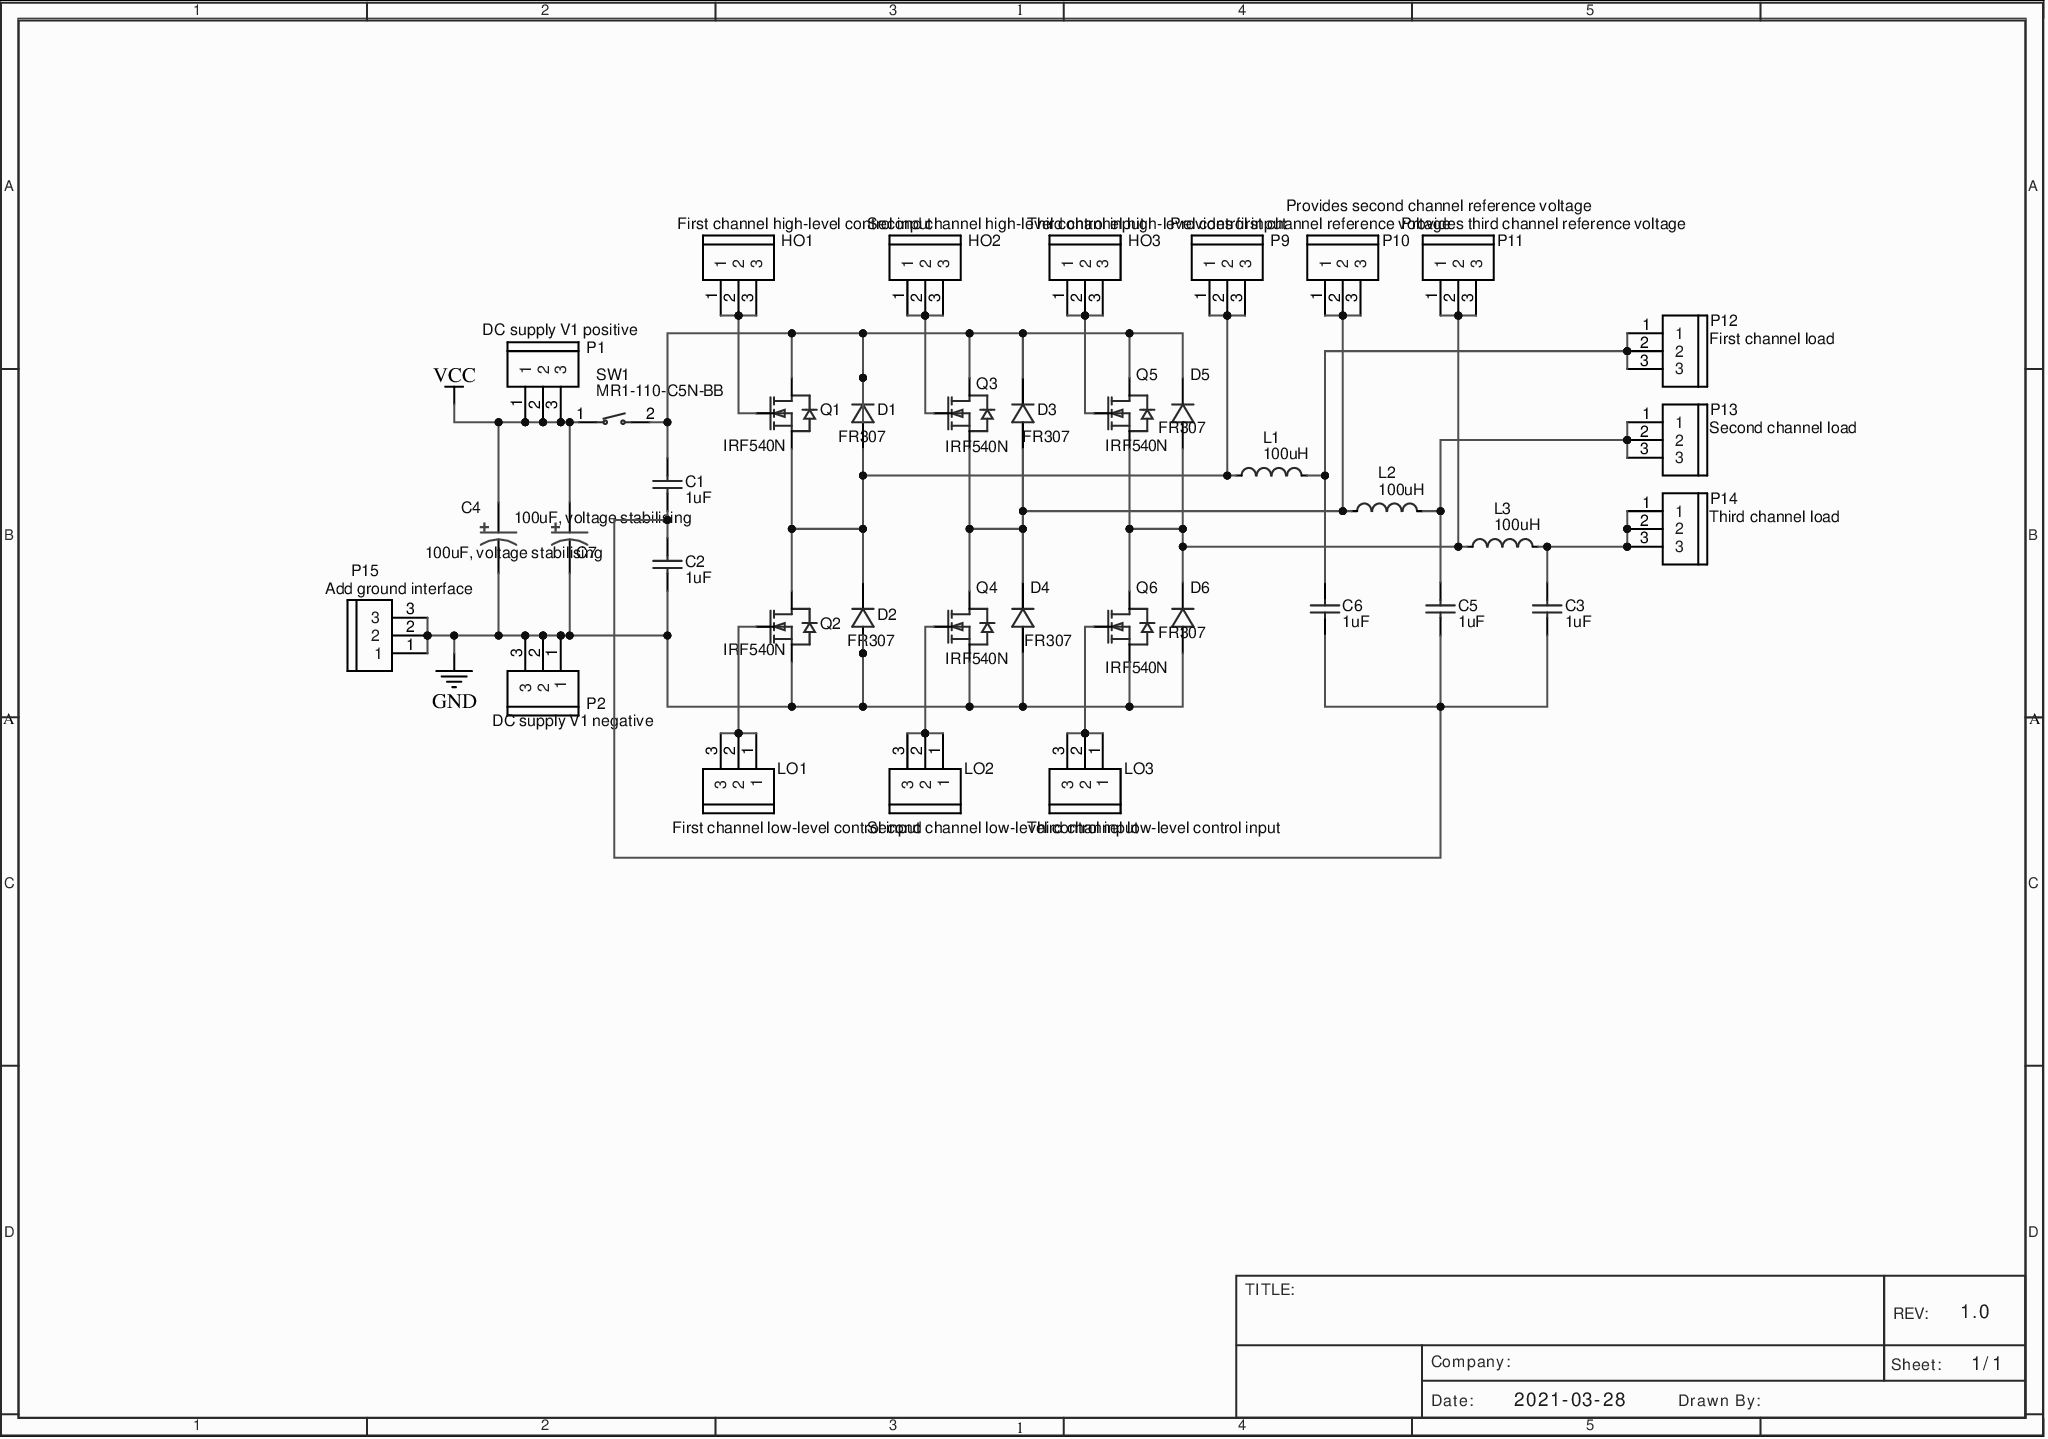
[diagram p0: MISC75150-3.schdoc]
# Altium project MISC75150-2.PrjPcb
1 sheet, 38 parts. Net scope: global (net labels, ports and power ports of the same name join across sheets).
Board file: MISC75150.pcbdoc

## Sheet MISC75150-3.schdoc
size 292 x 205 mm; Name: MISC75150; @Project Name: MISC75150; REV: 1.0; Date: 2021-03-28; Sheet: 1/1; Manufacturer Part: ?

### Parts
C1  1uF  [CAP-TH_L18.0-W9.5-P15.00-D1.2]
C2  1uF  [CAP-TH_L18.0-W9.5-P15.00-D1.2]
C3  1uF  [CAP-TH_L18.0-W9.5-P15.00-D1.2]
C4  100uF, voltage stabilising  [CAP-TH_BD8.0-P3.50-D1.0-FD]
C5  1uF  [CAP-TH_L18.0-W9.5-P15.00-D1.2]
C6  1uF  [CAP-TH_L18.0-W9.5-P15.00-D1.2]
C7  100uF, voltage stabilising  [CAP-TH_BD8.0-P3.50-D1.0-FD]
D1  FR307  [DO-201AD_BD5.3-L8.4-P12.50-D1.4-RD]
D2  FR307  [DO-201AD_BD5.3-L8.4-P12.50-D1.4-RD]
D3  FR307  [DO-201AD_BD5.3-L8.4-P12.50-D1.4-RD]
D4  FR307  [DO-201AD_BD5.3-L8.4-P12.50-D1.4-RD]
D5  FR307  [DO-201AD_BD5.3-L8.4-P12.50-D1.4-RD]
D6  FR307  [DO-201AD_BD5.3-L8.4-P12.50-D1.4-RD]
HO1  First channel high-level control input  [CONN-TH_3P-P5.00_WJ500V-5.08-3P]
HO2  Second channel high-level control input  [CONN-TH_3P-P5.00_WJ500V-5.08-3P]
HO3  Third channel high-level control input  [CONN-TH_3P-P5.00_WJ500V-5.08-3P]
L1  100uH  [IND-SMD_L13.5-W12.6_125CDMCC-DS]
L2  100uH  [IND-SMD_L13.5-W12.6_125CDMCC-DS]
L3  100uH  [IND-SMD_L13.5-W12.6_125CDMCC-DS]
LO1  First channel low-level control input  [CONN-TH_3P-P5.00_WJ500V-5.08-3P]
LO2  Second channel low-level control input  [CONN-TH_3P-P5.00_WJ500V-5.08-3P]
LO3  Third channel low-level control input  [CONN-TH_3P-P5.00_WJ500V-5.08-3P]
P1  DC supply V1 positive  [CONN-TH_3P-P5.00_WJ500V-5.08-3P]
P2  DC supply V1 negative  [CONN-TH_3P-P5.00_WJ500V-5.08-3P]
P9  Provides first channel reference voltage  [CONN-TH_3P-P5.00_WJ500V-5.08-3P]
P10  Provides second channel reference voltage  [CONN-TH_3P-P5.00_WJ500V-5.08-3P]
P11  Provides third channel reference voltage  [CONN-TH_3P-P5.00_WJ500V-5.08-3P]
P12  First channel load  [CONN-TH_3P-P5.00_WJ500V-5.08-3P]
P13  Second channel load  [CONN-TH_3P-P5.00_WJ500V-5.08-3P]
P14  Third channel load  [CONN-TH_3P-P5.00_WJ500V-5.08-3P]
P15  Add ground interface  [CONN-TH_3P-P5.00_WJ500V-5.08-3P]
Q1  IRF540N  [TO-220AB-3_L10.4-W4.6-P2.54-L]
Q2  IRF540N  [TO-220AB-3_L10.4-W4.6-P2.54-L]
Q3  IRF540N  [TO-220AB-3_L10.4-W4.6-P2.54-L]
Q4  IRF540N  [TO-220AB-3_L10.4-W4.6-P2.54-L]
Q5  IRF540N  [TO-220AB-3_L10.4-W4.6-P2.54-L]
Q6  IRF540N  [TO-220AB-3_L10.4-W4.6-P2.54-L]
SW1  MR1-110-C5N-BB  [SW-TH_MR1-110-C5N-BB]

### Nets
GND: C2.1 C4.2 C7.2 D2.2 D4.2 D6.2 P2.1 P2.2 P2.3 P15.1 P15.2 P15.3 Q2.3(S) Q4.3(S) Q6.3(S)
VCC: C4.1 C7.1 P1.1 P1.2 P1.3 SW1.1
NetC1_1: C1.1 C2.2 C3.1 C5.1 C6.1
NetC1_2: C1.2 D1.1 D3.1 D5.1 Q1.2(D) Q3.2(D) Q5.2(D) SW1.2
NetC3_2: C3.2 L3.2 P14.1 P14.2 P14.3
NetC5_2: C5.2 L2.2 P13.1 P13.2 P13.3
NetC6_2: C6.2 L1.2 P12.1 P12.2 P12.3
NetD1_2: D1.2 D2.1 L1.1 P9.1 P9.2 P9.3 Q1.3(S) Q2.2(D)
NetD3_2: D3.2 D4.1 L2.1 P10.1 P10.2 P10.3 Q3.3(S) Q4.2(D)
NetD5_2: D5.2 D6.1 L3.1 P11.1 P11.2 P11.3 Q5.3(S) Q6.2(D)
NetHO1_1: HO1.1 HO1.2 HO1.3 Q1.1(G)
NetHO2_1: HO2.1 HO2.2 HO2.3 Q3.1(G)
NetHO3_1: HO3.1 HO3.2 HO3.3 Q5.1(G)
NetLO1_1: LO1.1 LO1.2 LO1.3 Q2.1(G)
NetLO2_1: LO2.1 LO2.2 LO2.3 Q4.1(G)
NetLO3_1: LO3.1 LO3.2 LO3.3 Q6.1(G)

### Notes on the sheet
- 1
- 2
- 3
- 4
- 5
- A
- B
- C
- D
- TITLE:
- Company:
- Sheet:
- REV:
- 1.0
- 1/1
- Date:
- 2021-03-28
- Drawn By:

### Library data of the parts
C1 = ECWF2W105KA: Manufacturer: PANASONIC; Paste Type: expand; Convert to PCB: yes; UniqueId: ggee4a7045e9711cf46; OriginModelName: CAP-TH_L18.1-W9.3-H12.6-P15.0; ModelTransform: 712.597,366.141,0,0,0,0,0,0,-137.795; Device: ECWF2W105KA; Supplier: LCSC; Manufacturer Part: ECWF2W105KA; Supplier Part: C128505; Add into BOM: yes; SymbolName: 1uF; FootprintName: CAP-TH_L18.0-W9.5-P15.00-D1.2
C2 = ECWF2W105KA: Manufacturer: PANASONIC; Paste Type: expand; Convert to PCB: yes; UniqueId: gge8b30a07ac08630fb; OriginModelName: CAP-TH_L18.1-W9.3-H12.6-P15.0; ModelTransform: 712.597,366.141,0,0,0,0,0,0,-137.795; Device: ECWF2W105KA; Supplier: LCSC; Manufacturer Part: ECWF2W105KA; Supplier Part: C128505; Add into BOM: yes; SymbolName: 1uF; FootprintName: CAP-TH_L18.0-W9.5-P15.00-D1.2
C3 = ECWF2W105KA: Manufacturer: PANASONIC; Paste Type: expand; Convert to PCB: yes; UniqueId: ggeb8cf41ff4f0b6587; OriginModelName: CAP-TH_L18.1-W9.3-H12.6-P15.0; ModelTransform: 712.597,366.141,0,0,0,0,0,0,-137.795; Device: ECWF2W105KA; Supplier: LCSC; Manufacturer Part: ECWF2W105KA; Supplier Part: C128505; Add into BOM: yes; SymbolName: 1uF; FootprintName: CAP-TH_L18.0-W9.5-P15.00-D1.2
C4 = SPV1HM101F11O00RAXXX: Manufacturer: Aihua Group; Convert to PCB: yes; UniqueId: ggee92f5958b3224aee; OriginModelName: CAP-TH_D8.0-H8.0-P3.50; ModelTransform: 314.96,314.862,0,180,0,0,0,0,-118.11; Device: SPV1HM101F11O00RAXXX; Supplier: LCSC; Supplier Part: C167234; Manufacturer Part: SPV1HM101F11O00RAXXX; Add into BOM: yes; SymbolName: 100uF, voltage stabilising; FootprintName: CAP-TH_BD8.0-P3.50-D1.0-FD
C5 = ECWF2W105KA: Manufacturer: PANASONIC; Paste Type: expand; Convert to PCB: yes; UniqueId: gge1386f1878ac6b3a8; OriginModelName: CAP-TH_L18.1-W9.3-H12.6-P15.0; ModelTransform: 712.597,366.141,0,0,0,0,0,0,-137.795; Device: ECWF2W105KA; Supplier: LCSC; Manufacturer Part: ECWF2W105KA; Supplier Part: C128505; Add into BOM: yes; SymbolName: 1uF; FootprintName: CAP-TH_L18.0-W9.5-P15.00-D1.2
C6 = ECWF2W105KA: Manufacturer: PANASONIC; Paste Type: expand; Convert to PCB: yes; UniqueId: gge8976a15bcc07fff3; OriginModelName: CAP-TH_L18.1-W9.3-H12.6-P15.0; ModelTransform: 712.597,366.141,0,0,0,0,0,0,-137.795; Device: ECWF2W105KA; Supplier: LCSC; Manufacturer Part: ECWF2W105KA; Supplier Part: C128505; Add into BOM: yes; SymbolName: 1uF; FootprintName: CAP-TH_L18.0-W9.5-P15.00-D1.2
C7 = SPV1HM101F11O00RAXXX: Manufacturer: Aihua Group; Convert to PCB: yes; UniqueId: ggeb1f74c670b6129be; OriginModelName: CAP-TH_D8.0-H8.0-P3.50; ModelTransform: 314.96,314.862,0,180,0,0,0,0,-118.11; Device: SPV1HM101F11O00RAXXX; Supplier: LCSC; Supplier Part: C167234; Manufacturer Part: SPV1HM101F11O00RAXXX; Add into BOM: yes; SymbolName: 100uF, voltage stabilising; FootprintName: CAP-TH_BD8.0-P3.50-D1.0-FD
D1 = FR307: Manufacturer: Yangzhou Yangjie Elec Tech; Paste Type: expand; Convert to PCB: yes; UniqueId: gge83b63f64a46c2831; OriginModelName: DO-201AD_D5.3-L8.4-P13.6; ModelTransform: 582.676,208.5295,0,0,0,0,0,0,-137.795; Device: FR307; Supplier: LCSC; Supplier Part: C698674; Manufacturer Part: FR307; Add into BOM: yes; SymbolName: FR307; FootprintName: DO-201AD_BD5.3-L8.4-P12.50-D1.4-RD
D2 = FR307: Manufacturer: Yangzhou Yangjie Elec Tech; Paste Type: expand; Convert to PCB: yes; UniqueId: ggea2ef0e735770ea0f; OriginModelName: DO-201AD_D5.3-L8.4-P13.6; ModelTransform: 582.676,208.5295,0,0,0,0,0,0,-137.795; Device: FR307; Supplier: LCSC; Supplier Part: C698674; Manufacturer Part: FR307; Add into BOM: yes; SymbolName: FR307; FootprintName: DO-201AD_BD5.3-L8.4-P12.50-D1.4-RD
D3 = FR307: Manufacturer: Yangzhou Yangjie Elec Tech; Paste Type: expand; Convert to PCB: yes; UniqueId: ggeac6837f34457c33d; OriginModelName: DO-201AD_D5.3-L8.4-P13.6; ModelTransform: 582.676,208.5295,0,0,0,0,0,0,-137.795; Device: FR307; Supplier: LCSC; Supplier Part: C698674; Manufacturer Part: FR307; Add into BOM: yes; SymbolName: FR307; FootprintName: DO-201AD_BD5.3-L8.4-P12.50-D1.4-RD
D4 = FR307: Manufacturer: Yangzhou Yangjie Elec Tech; Paste Type: expand; Convert to PCB: yes; UniqueId: gge96a78163855c4fac; OriginModelName: DO-201AD_D5.3-L8.4-P13.6; ModelTransform: 582.676,208.5295,0,0,0,0,0,0,-137.795; Device: FR307; Supplier: LCSC; Supplier Part: C698674; Manufacturer Part: FR307; Add into BOM: yes; SymbolName: FR307; FootprintName: DO-201AD_BD5.3-L8.4-P12.50-D1.4-RD
D5 = FR307: Manufacturer: Yangzhou Yangjie Elec Tech; Paste Type: expand; Convert to PCB: yes; UniqueId: gge21288790032872b2; OriginModelName: DO-201AD_D5.3-L8.4-P13.6; ModelTransform: 582.676,208.5295,0,0,0,0,0,0,-137.795; Device: FR307; Supplier: LCSC; Supplier Part: C698674; Manufacturer Part: FR307; Add into BOM: yes; SymbolName: FR307; FootprintName: DO-201AD_BD5.3-L8.4-P12.50-D1.4-RD
D6 = FR307: Manufacturer: Yangzhou Yangjie Elec Tech; Paste Type: expand; Convert to PCB: yes; UniqueId: gge82c1ee6ae88ddc6b; OriginModelName: DO-201AD_D5.3-L8.4-P13.6; ModelTransform: 582.676,208.5295,0,0,0,0,0,0,-137.795; Device: FR307; Supplier: LCSC; Supplier Part: C698674; Manufacturer Part: FR307; Add into BOM: yes; SymbolName: FR307; FootprintName: DO-201AD_BD5.3-L8.4-P12.50-D1.4-RD
HO1 = WJ500V-5.08-3P-14-00A: Manufacturer: ReliaPro; Paste Type: expand; Convert to PCB: yes; UniqueId: gge2b5cea29c56c81ac; OriginModelName: CONN-TH_3P_L15.3-W10.2-P5.08; ModelTransform: 619.674,413.385,0,0,0,0,-7.874,0,-157.48; Device: WJ500V-5.08-3P-14-00A; Supplier: LCSC; Manufacturer Part: WJ500V-5.08-3P-14-00A; image: C72334.jpg; Supplier Part: C72334; Add into BOM: yes; SymbolName: First channel high-level control input; FootprintName: CONN-TH_3P-P5.00_WJ500V-5.08-3P
HO2 = WJ500V-5.08-3P-14-00A: Manufacturer: ReliaPro; Paste Type: expand; Convert to PCB: yes; UniqueId: gge3b87de472fa51f12; OriginModelName: CONN-TH_3P_L15.3-W10.2-P5.08; ModelTransform: 619.674,413.385,0,0,0,0,-7.874,0,-157.48; Device: WJ500V-5.08-3P-14-00A; Supplier: LCSC; Manufacturer Part: WJ500V-5.08-3P-14-00A; image: C72334.jpg; Supplier Part: C72334; Add into BOM: yes; SymbolName: Second channel high-level control input; FootprintName: CONN-TH_3P-P5.00_WJ500V-5.08-3P
HO3 = WJ500V-5.08-3P-14-00A: Manufacturer: ReliaPro; Paste Type: expand; Convert to PCB: yes; UniqueId: ggef853e3d0681c0b1a; OriginModelName: CONN-TH_3P_L15.3-W10.2-P5.08; ModelTransform: 619.674,413.385,0,0,0,0,-7.874,0,-157.48; Device: WJ500V-5.08-3P-14-00A; Supplier: LCSC; Manufacturer Part: WJ500V-5.08-3P-14-00A; image: C72334.jpg; Supplier Part: C72334; Add into BOM: yes; SymbolName: Third channel high-level control input; FootprintName: CONN-TH_3P-P5.00_WJ500V-5.08-3P
L1 = TMPC1206HP-101MG-D: Manufacturer: TAITEC; Convert to PCB: yes; UniqueId: gged90d88dc2415983d; OriginModelName: IND-SMD_L13.5-W12.6-H5.7; ModelTransform: 531.495,492.125,0,0,0,0,0,0,0; Device: TMPC1206HP-101MG-D; Supplier: LCSC; Supplier Part: C357256; Manufacturer Part: TMPC1206HP-101MG-D; Add into BOM: yes; SymbolName: 100uH; FootprintName: IND-SMD_L13.5-W12.6_125CDMCC-DS
L2 = TMPC1206HP-101MG-D: Manufacturer: TAITEC; Convert to PCB: yes; UniqueId: ggeadd428e7fae9a274; OriginModelName: IND-SMD_L13.5-W12.6-H5.7; ModelTransform: 531.495,492.125,0,0,0,0,0,0,0; Device: TMPC1206HP-101MG-D; Supplier: LCSC; Supplier Part: C357256; Manufacturer Part: TMPC1206HP-101MG-D; Add into BOM: yes; SymbolName: 100uH; FootprintName: IND-SMD_L13.5-W12.6_125CDMCC-DS
L3 = TMPC1206HP-101MG-D: Manufacturer: TAITEC; Convert to PCB: yes; UniqueId: ggeea68f54d1f5691be; OriginModelName: IND-SMD_L13.5-W12.6-H5.7; ModelTransform: 531.495,492.125,0,0,0,0,0,0,0; Device: TMPC1206HP-101MG-D; Supplier: LCSC; Supplier Part: C357256; Manufacturer Part: TMPC1206HP-101MG-D; Add into BOM: yes; SymbolName: 100uH; FootprintName: IND-SMD_L13.5-W12.6_125CDMCC-DS
LO1 = WJ500V-5.08-3P-14-00A: Manufacturer: ReliaPro; Paste Type: expand; Convert to PCB: yes; UniqueId: gge8d9840f4034438ff; OriginModelName: CONN-TH_3P_L15.3-W10.2-P5.08; ModelTransform: 619.674,413.385,0,0,0,0,-7.874,0,-157.48; Device: WJ500V-5.08-3P-14-00A; Supplier: LCSC; Manufacturer Part: WJ500V-5.08-3P-14-00A; image: C72334.jpg; Supplier Part: C72334; Add into BOM: yes; SymbolName: First channel low-level control input; FootprintName: CONN-TH_3P-P5.00_WJ500V-5.08-3P
LO2 = WJ500V-5.08-3P-14-00A: Manufacturer: ReliaPro; Paste Type: expand; Convert to PCB: yes; UniqueId: gge5f0c870194b11f33; OriginModelName: CONN-TH_3P_L15.3-W10.2-P5.08; ModelTransform: 619.674,413.385,0,0,0,0,-7.874,0,-157.48; Device: WJ500V-5.08-3P-14-00A; Supplier: LCSC; Manufacturer Part: WJ500V-5.08-3P-14-00A; image: C72334.jpg; Supplier Part: C72334; Add into BOM: yes; SymbolName: Second channel low-level control input; FootprintName: CONN-TH_3P-P5.00_WJ500V-5.08-3P
LO3 = WJ500V-5.08-3P-14-00A: Manufacturer: ReliaPro; Paste Type: expand; Convert to PCB: yes; UniqueId: gge96ab42e47ac765f7; OriginModelName: CONN-TH_3P_L15.3-W10.2-P5.08; ModelTransform: 619.674,413.385,0,0,0,0,-7.874,0,-157.48; Device: WJ500V-5.08-3P-14-00A; Supplier: LCSC; Manufacturer Part: WJ500V-5.08-3P-14-00A; image: C72334.jpg; Supplier Part: C72334; Add into BOM: yes; SymbolName: Third channel low-level control input; FootprintName: CONN-TH_3P-P5.00_WJ500V-5.08-3P
P1 = WJ500V-5.08-3P-14-00A: Manufacturer: ReliaPro; Paste Type: expand; Convert to PCB: yes; UniqueId: ggea21f75b8c584c3ca; OriginModelName: CONN-TH_3P_L15.3-W10.2-P5.08; ModelTransform: 619.674,413.385,0,0,0,0,-7.874,0,-157.48; Device: WJ500V-5.08-3P-14-00A; Supplier: LCSC; Manufacturer Part: WJ500V-5.08-3P-14-00A; image: C72334.jpg; Supplier Part: C72334; Add into BOM: yes; SymbolName: DC supply V1 positive; FootprintName: CONN-TH_3P-P5.00_WJ500V-5.08-3P
P2 = WJ500V-5.08-3P-14-00A: Manufacturer: ReliaPro; Paste Type: expand; Convert to PCB: yes; UniqueId: ggedf937a3e08b3b14d; OriginModelName: CONN-TH_3P_L15.3-W10.2-P5.08; ModelTransform: 619.674,413.385,0,0,0,0,-7.874,0,-157.48; Device: WJ500V-5.08-3P-14-00A; Supplier: LCSC; Manufacturer Part: WJ500V-5.08-3P-14-00A; image: C72334.jpg; Supplier Part: C72334; Add into BOM: yes; SymbolName: DC supply V1 negative; FootprintName: CONN-TH_3P-P5.00_WJ500V-5.08-3P
P9 = WJ500V-5.08-3P-14-00A: Manufacturer: ReliaPro; Paste Type: expand; Convert to PCB: yes; UniqueId: gge32828030546481a2; OriginModelName: CONN-TH_3P_L15.3-W10.2-P5.08; ModelTransform: 619.674,413.385,0,0,0,0,-7.874,0,-157.48; Device: WJ500V-5.08-3P-14-00A; Supplier: LCSC; Manufacturer Part: WJ500V-5.08-3P-14-00A; image: C72334.jpg; Supplier Part: C72334; Add into BOM: yes; SymbolName: Provides first channel reference voltage; FootprintName: CONN-TH_3P-P5.00_WJ500V-5.08-3P
P10 = WJ500V-5.08-3P-14-00A: Manufacturer: ReliaPro; Paste Type: expand; Convert to PCB: yes; UniqueId: gge041070466fecb40b; OriginModelName: CONN-TH_3P_L15.3-W10.2-P5.08; ModelTransform: 619.674,413.385,0,0,0,0,-7.874,0,-157.48; Device: WJ500V-5.08-3P-14-00A; Supplier: LCSC; Manufacturer Part: WJ500V-5.08-3P-14-00A; image: C72334.jpg; Supplier Part: C72334; Add into BOM: yes; SymbolName: Provides second channel reference voltage; FootprintName: CONN-TH_3P-P5.00_WJ500V-5.08-3P
P11 = WJ500V-5.08-3P-14-00A: Manufacturer: ReliaPro; Paste Type: expand; Convert to PCB: yes; UniqueId: gge2be2aeeb845be86a; OriginModelName: CONN-TH_3P_L15.3-W10.2-P5.08; ModelTransform: 619.674,413.385,0,0,0,0,-7.874,0,-157.48; Device: WJ500V-5.08-3P-14-00A; Supplier: LCSC; Manufacturer Part: WJ500V-5.08-3P-14-00A; image: C72334.jpg; Supplier Part: C72334; Add into BOM: yes; SymbolName: Provides third channel reference voltage; FootprintName: CONN-TH_3P-P5.00_WJ500V-5.08-3P
P12 = WJ500V-5.08-3P-14-00A: Manufacturer: ReliaPro; Paste Type: expand; Convert to PCB: yes; UniqueId: gge57af53ecf236b9ba; OriginModelName: CONN-TH_3P_L15.3-W10.2-P5.08; ModelTransform: 619.674,413.385,0,0,0,0,-7.874,0,-157.48; Device: WJ500V-5.08-3P-14-00A; Supplier: LCSC; Manufacturer Part: WJ500V-5.08-3P-14-00A; image: C72334.jpg; Supplier Part: C72334; Add into BOM: yes; SymbolName: First channel load; FootprintName: CONN-TH_3P-P5.00_WJ500V-5.08-3P
P13 = WJ500V-5.08-3P-14-00A: Manufacturer: ReliaPro; Paste Type: expand; Convert to PCB: yes; UniqueId: gge15ca11e844af06e8; OriginModelName: CONN-TH_3P_L15.3-W10.2-P5.08; ModelTransform: 619.674,413.385,0,0,0,0,-7.874,0,-157.48; Device: WJ500V-5.08-3P-14-00A; Supplier: LCSC; Manufacturer Part: WJ500V-5.08-3P-14-00A; image: C72334.jpg; Supplier Part: C72334; Add into BOM: yes; SymbolName: Second channel load; FootprintName: CONN-TH_3P-P5.00_WJ500V-5.08-3P
P14 = WJ500V-5.08-3P-14-00A: Manufacturer: ReliaPro; Paste Type: expand; Convert to PCB: yes; UniqueId: gge8e9976c4e9bbe8ab; OriginModelName: CONN-TH_3P_L15.3-W10.2-P5.08; ModelTransform: 619.674,413.385,0,0,0,0,-7.874,0,-157.48; Device: WJ500V-5.08-3P-14-00A; Supplier: LCSC; Manufacturer Part: WJ500V-5.08-3P-14-00A; image: C72334.jpg; Supplier Part: C72334; Add into BOM: yes; SymbolName: Third channel load; FootprintName: CONN-TH_3P-P5.00_WJ500V-5.08-3P
P15 = WJ500V-5.08-3P-14-00A: Manufacturer: ReliaPro; Paste Type: expand; Convert to PCB: yes; UniqueId: gge32ca391a8d4bf8ce; OriginModelName: CONN-TH_3P_L15.3-W10.2-P5.08; ModelTransform: 619.674,413.385,0,0,0,0,-7.874,0,-157.48; Device: WJ500V-5.08-3P-14-00A; Supplier: LCSC; Manufacturer Part: WJ500V-5.08-3P-14-00A; image: C72334.jpg; Supplier Part: C72334; Add into BOM: yes; SymbolName: Add ground interface; FootprintName: CONN-TH_3P-P5.00_WJ500V-5.08-3P
Q1 = IRF540N: Manufacturer: VBsemi Elec; Paste Type: expand; Convert to PCB: yes; UniqueId: ggecc56a0e218d81875; OriginModelName: TO-220AB_3PIN-L10.5-W5.0-H20.0-P2.54; ModelTransform: 413.385,191.3382,0,0,0,0,0,25.591,-393.701; Device: IRF540N; Supplier: LCSC; Supplier Part: C693382; Manufacturer Part: IRF540N; Add into BOM: yes; SymbolName: IRF540N; FootprintName: TO-220AB-3_L10.4-W4.6-P2.54-L
Q2 = IRF540N: Manufacturer: VBsemi Elec; Paste Type: expand; Convert to PCB: yes; UniqueId: gge57153b100eafbdc0; OriginModelName: TO-220AB_3PIN-L10.5-W5.0-H20.0-P2.54; ModelTransform: 413.385,191.3382,0,0,0,0,0,25.591,-393.701; Device: IRF540N; Supplier: LCSC; Supplier Part: C693382; Manufacturer Part: IRF540N; Add into BOM: yes; SymbolName: IRF540N; FootprintName: TO-220AB-3_L10.4-W4.6-P2.54-L
Q3 = IRF540N: Manufacturer: VBsemi Elec; Paste Type: expand; Convert to PCB: yes; UniqueId: gge06dfc0ecad9b2168; OriginModelName: TO-220AB_3PIN-L10.5-W5.0-H20.0-P2.54; ModelTransform: 413.385,191.3382,0,0,0,0,0,25.591,-393.701; Device: IRF540N; Supplier: LCSC; Supplier Part: C693382; Manufacturer Part: IRF540N; Add into BOM: yes; SymbolName: IRF540N; FootprintName: TO-220AB-3_L10.4-W4.6-P2.54-L
Q4 = IRF540N: Manufacturer: VBsemi Elec; Paste Type: expand; Convert to PCB: yes; UniqueId: ggec4d9214183939f34; OriginModelName: TO-220AB_3PIN-L10.5-W5.0-H20.0-P2.54; ModelTransform: 413.385,191.3382,0,0,0,0,0,25.591,-393.701; Device: IRF540N; Supplier: LCSC; Supplier Part: C693382; Manufacturer Part: IRF540N; Add into BOM: yes; SymbolName: IRF540N; FootprintName: TO-220AB-3_L10.4-W4.6-P2.54-L
Q5 = IRF540N: Manufacturer: VBsemi Elec; Paste Type: expand; Convert to PCB: yes; UniqueId: ggea1b8e10c3745224e; OriginModelName: TO-220AB_3PIN-L10.5-W5.0-H20.0-P2.54; ModelTransform: 413.385,191.3382,0,0,0,0,0,25.591,-393.701; Device: IRF540N; Supplier: LCSC; Supplier Part: C693382; Manufacturer Part: IRF540N; Add into BOM: yes; SymbolName: IRF540N; FootprintName: TO-220AB-3_L10.4-W4.6-P2.54-L
Q6 = IRF540N: Manufacturer: VBsemi Elec; Paste Type: expand; Convert to PCB: yes; UniqueId: gge1d368d93c2e32122; OriginModelName: TO-220AB_3PIN-L10.5-W5.0-H20.0-P2.54; ModelTransform: 413.385,191.3382,0,0,0,0,0,25.591,-393.701; Device: IRF540N; Supplier: LCSC; Supplier Part: C693382; Manufacturer Part: IRF540N; Add into BOM: yes; SymbolName: IRF540N; FootprintName: TO-220AB-3_L10.4-W4.6-P2.54-L
SW1 = MR1-110-C5N-BB: Manufacturer: HONGJU; Paste Type: expand; Convert to PCB: yes; UniqueId: gge3bbf4f6bb6262bb3; Device: MR1-110-C5N-BB; Supplier: LCSC; Supplier Part: C268222; Manufacturer Part: MR1-110-C5N-BB; Add into BOM: yes; SymbolName: MR1-110-C5N-BB; FootprintName: SW-TH_MR1-110-C5N-BB